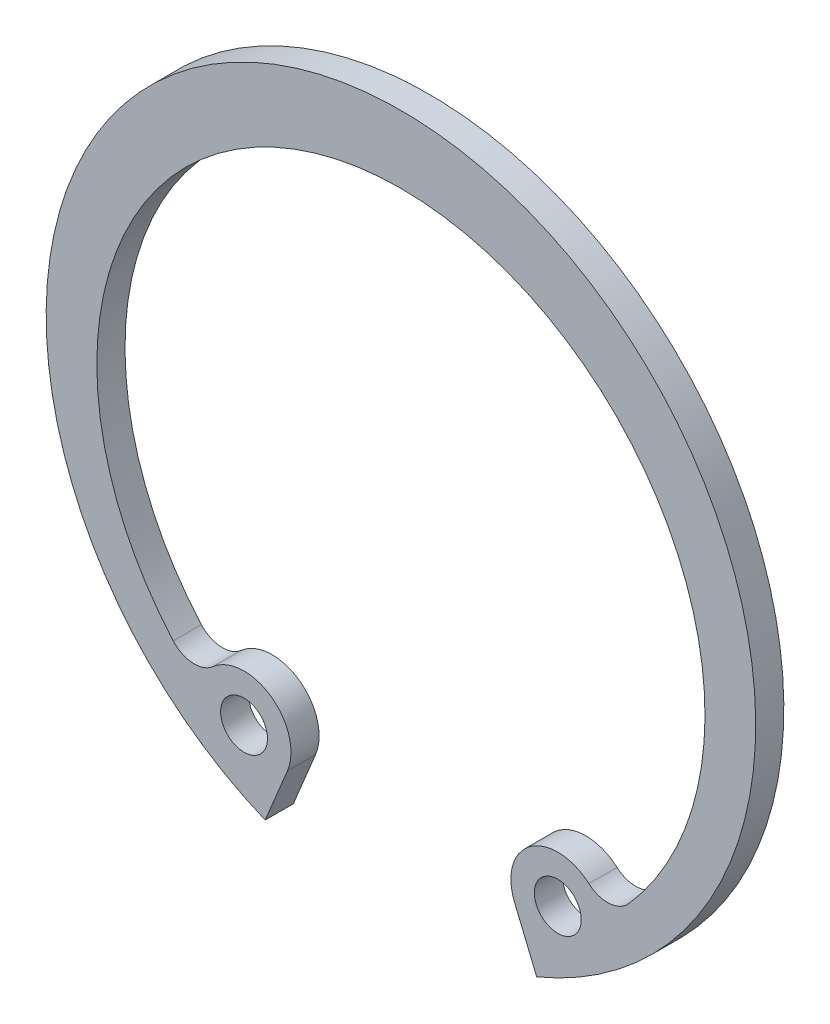
SolidWorks part; units mm, degrees
ref_plane "Front" through (0, 0, 0) normal (0, 0, 1) x (1, 0, 0)
ref_plane "Top" through (0, 0, 0) normal (0, 1, 0) x (1, 0, 0)
ref_plane "Right" through (0, 0, 0) normal (1, 0, 0) x (0, 0, -1)
sketch "Sketch1" plane through (0, 0, 0) normal (0, 0, 1) x (1, 0, 0)
  line L0 (0, 0) -> (-6.0477, -14.6005) construction
  line L1 (0, 7.3554) -> (0, -7.1505) construction
  line L2 (6.0477, -14.6005) -> (7.2327, -17.4613)
  line L4 (-6.0477, -14.6005) -> (-7.2327, -17.4613)
  arc A0 (7.2327, -17.4613) -> (-7.2327, -17.4613) centre (0, 0) ccw
  arc A1 (12.1282, -11.64) -> (-12.1282, -11.64) centre (0, -0.9) ccw
  arc A2 (-6.0477, -14.6005) -> (-10.0123, -11.7699) centre (-8.3574, -13.6438) ccw
  arc A3 (-12.1282, -11.64) -> (-10.0123, -11.7699) centre (-11.0052, -10.6456) ccw
  circle A4 centre (8.3574, -13.6438) radius 1.25
  arc A5 (12.1282, -11.64) -> (10.0123, -11.7699) centre (11.0052, -10.6456) cw
  arc A6 (-16, 0) -> (16, 0) centre (0, 0) ccw construction
  circle A7 centre (-8.3574, -13.6438) radius 1.25
  arc A8 (6.0477, -14.6005) -> (10.0123, -11.7699) centre (8.3574, -13.6438) cw
  dimension "D" = 37.8
  dimension "d0" = 32.4
  dimension "R1" = 2.5
  dimension "R2" = 1.5
  dimension "d1" = 2.5
  dimension "R" = 16
  dimension "C" = 0.9
  dimension "Angle" = 45
extrude "Body" add sketch "Sketch1" against normal blind 1.5
